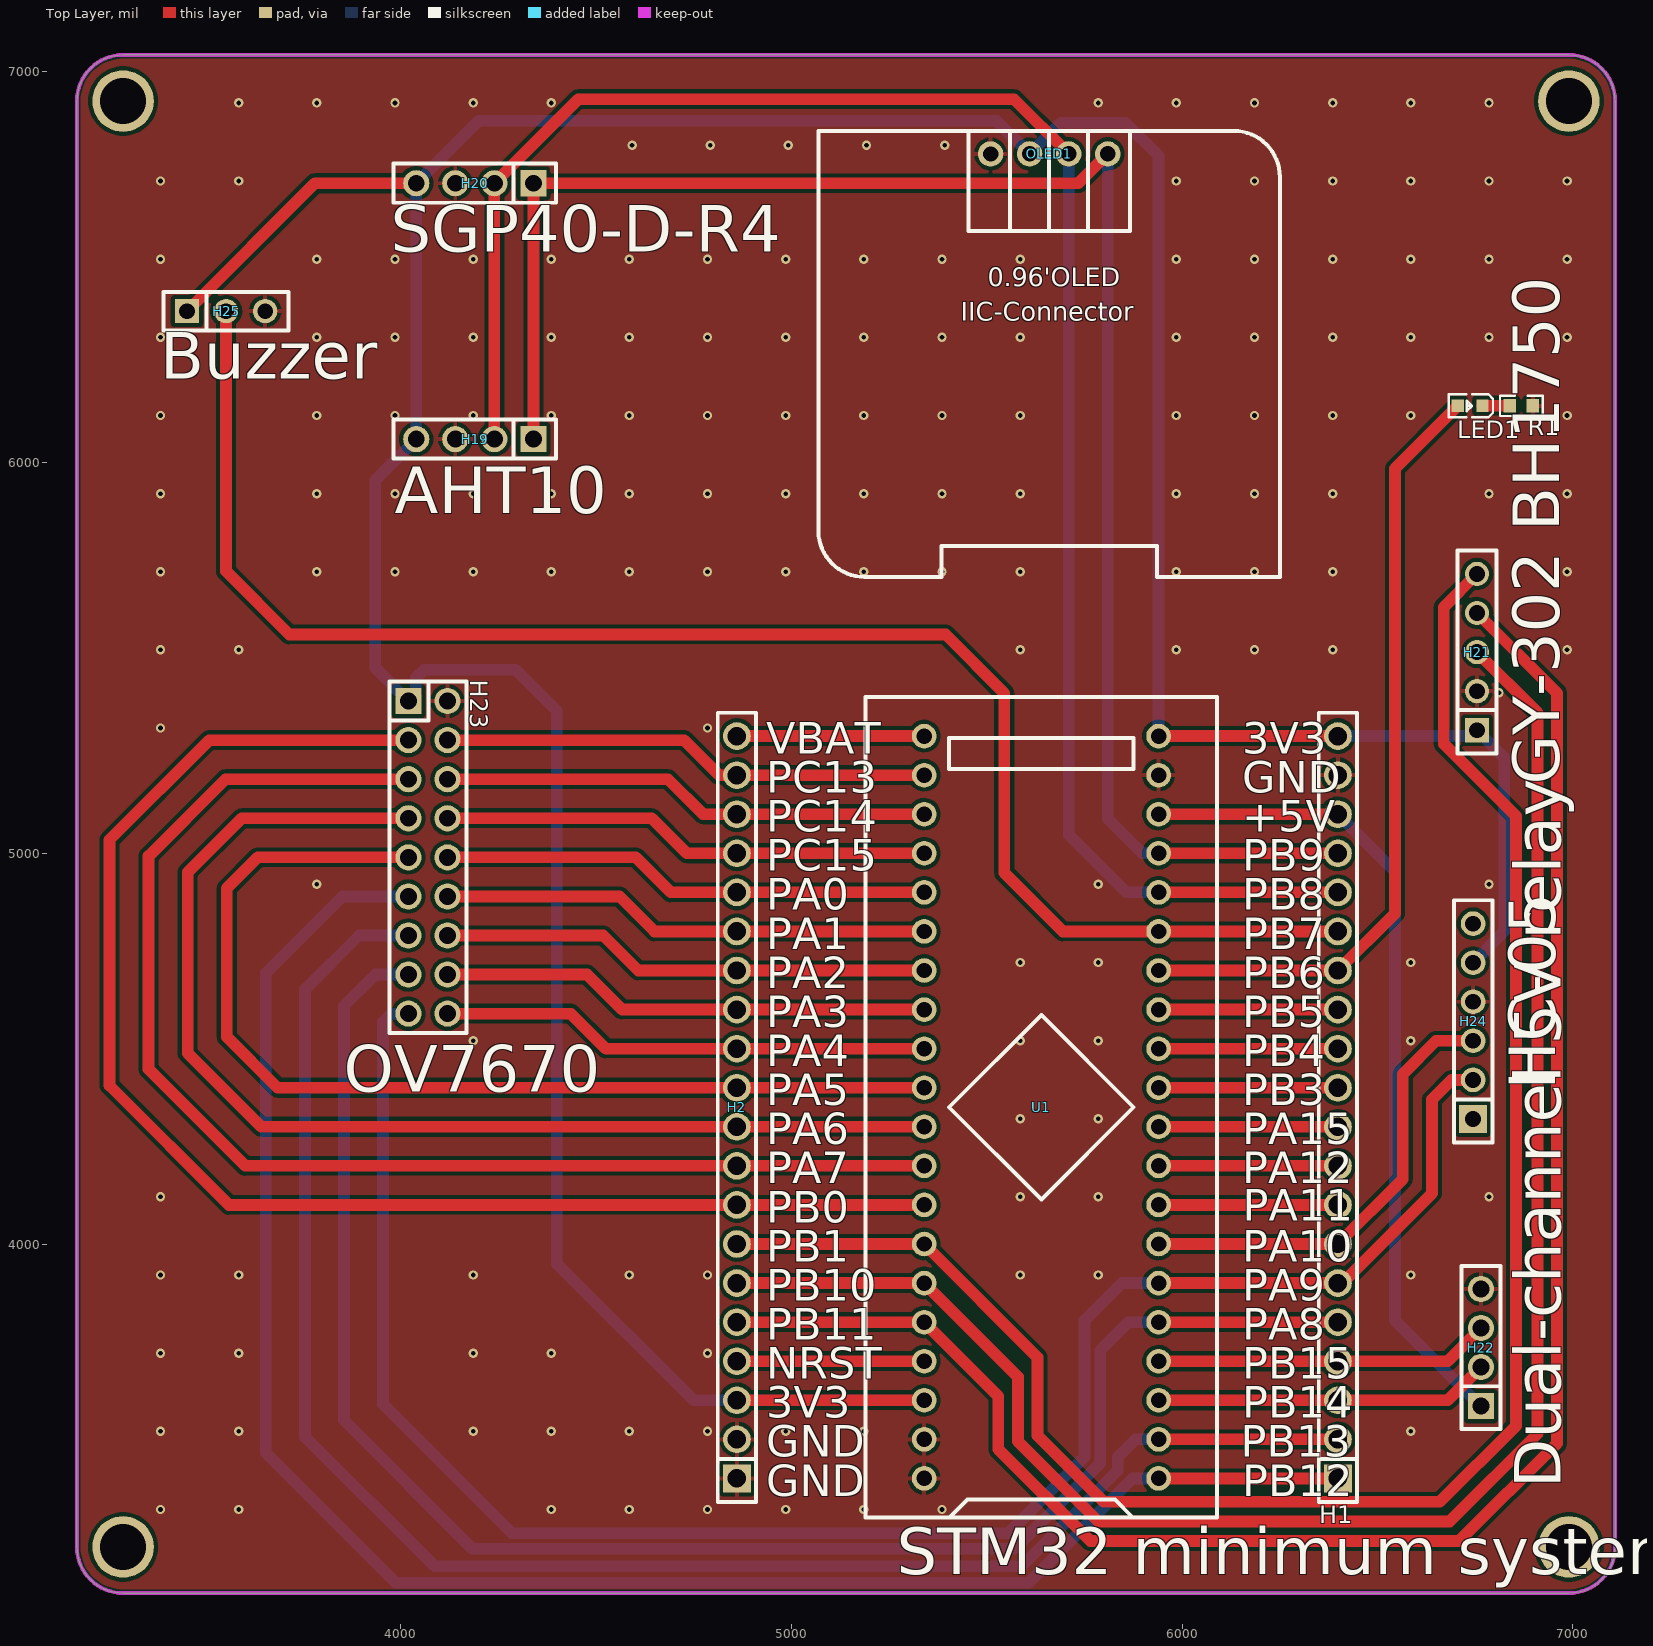
[diagram p0: Top Layer view]
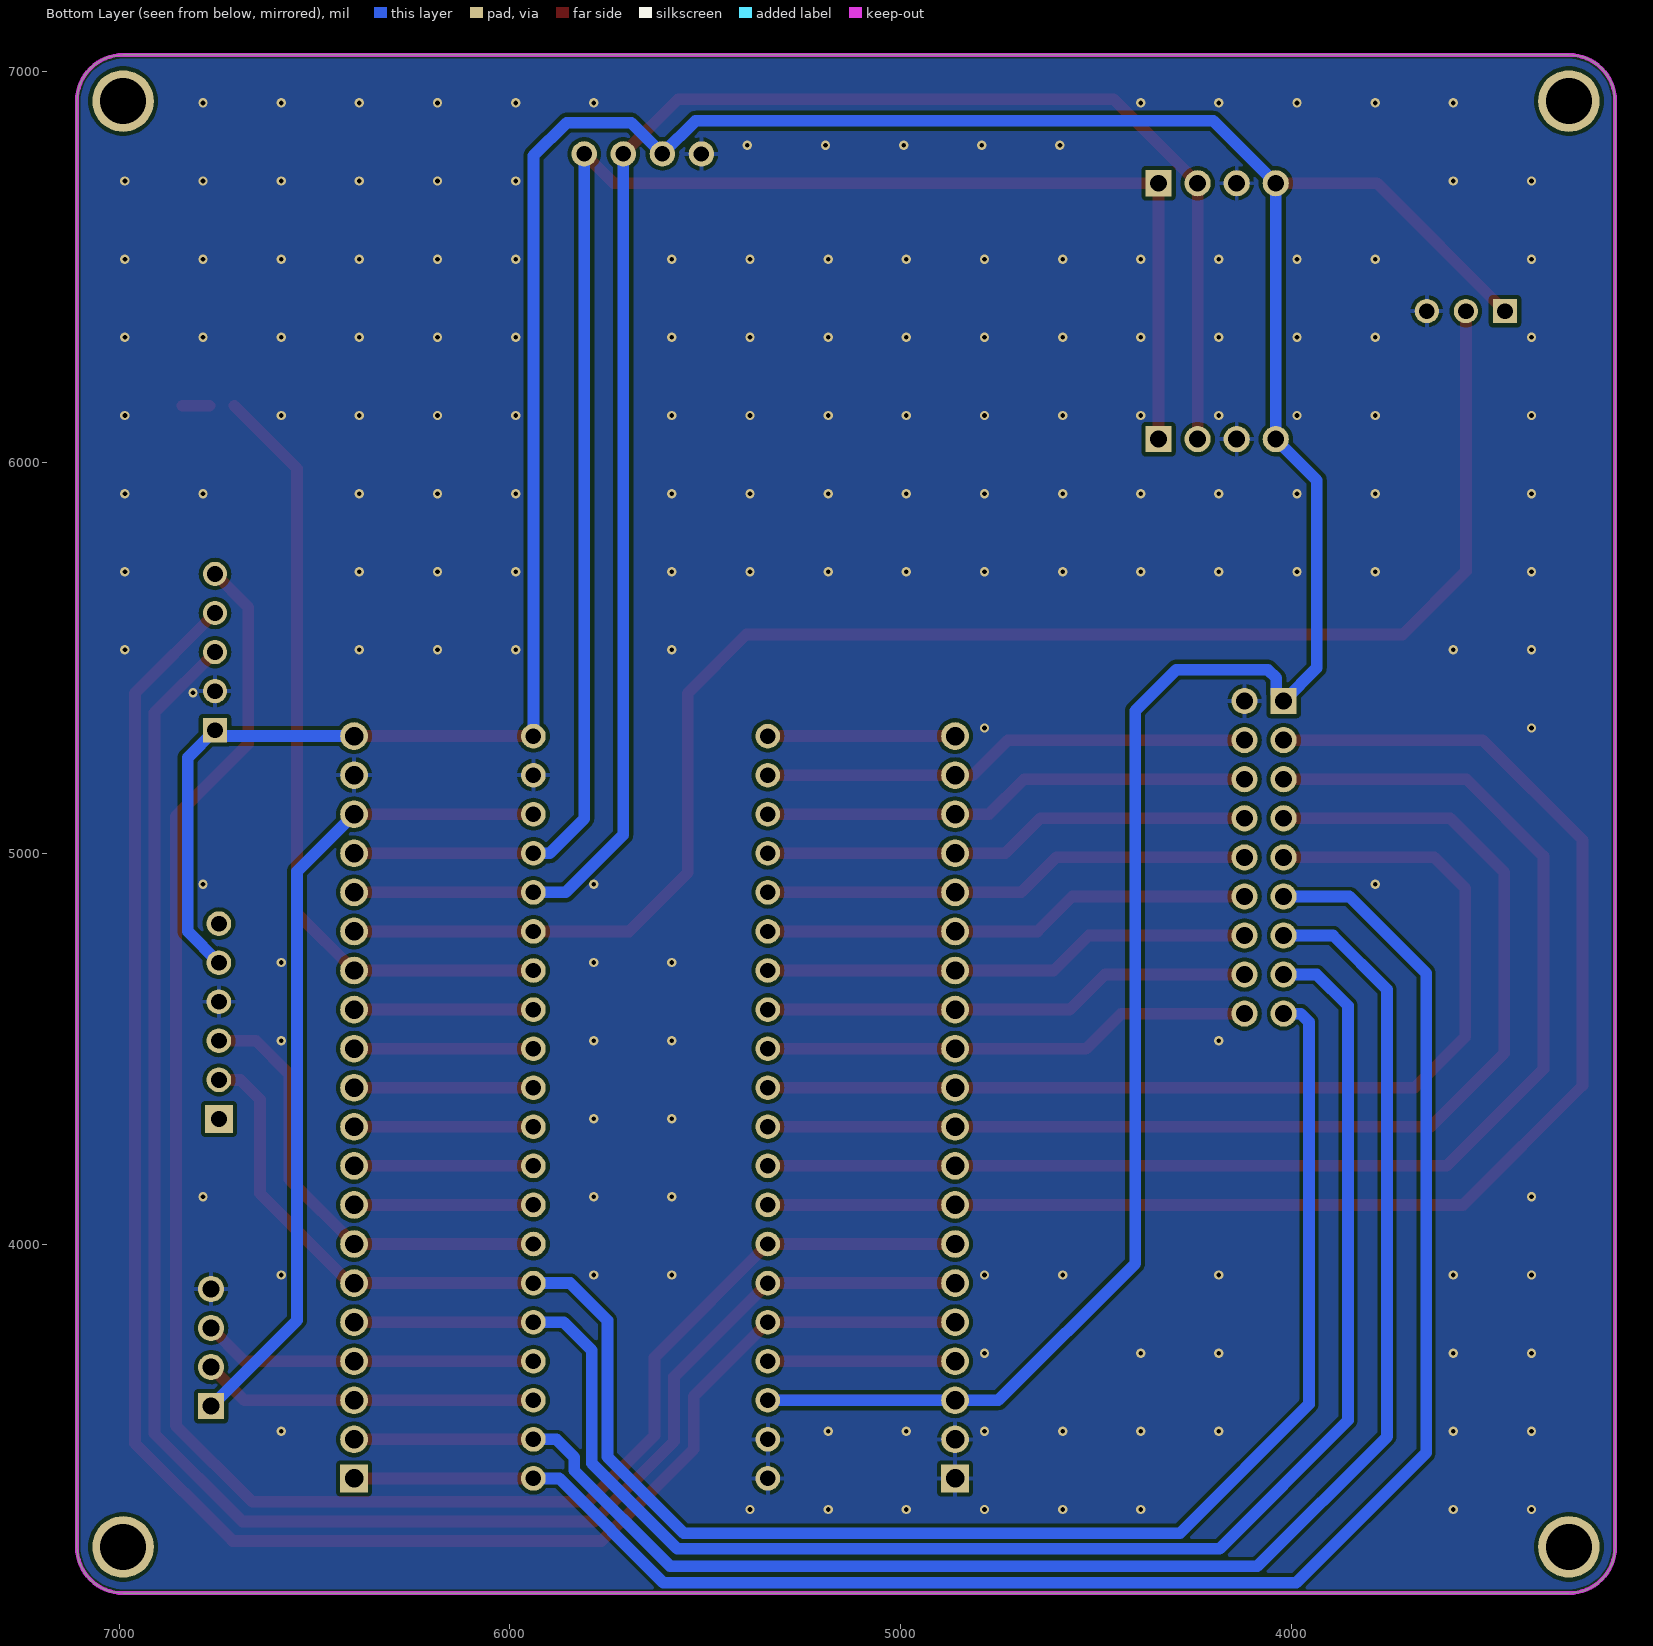
[diagram p1: Bottom Layer view, seen from below]
# Altium PCB MISC78996.pcbdoc
Units mil, origin at the board's own origin, x right, y up, seen from the top; angles counter-clockwise.
Board outline 3937.01 x 3937.01 mil, 2 copper layers (Top Layer, Bottom Layer), stack 62.206 mil thick; 13 components, 38 nets, 136 pads, 161 vias.

## Layer stack, top to bottom
Top Solder Mask Layer: solder mask 0.394, Dk 3.3
Top Layer: signal copper 1.379
Dielectric1: surface 59.449, FR4, Dk 4.5
Bottom Layer: signal copper 1.378
Bottom Solder Mask Layer: solder mask 0.394, Dk 3.3

## Board outline
3289.61,7043.5 ccw(c3289.61,6925.39) 3171.5,6925.39 3171.5,3224.61 ccw(c3289.61,3224.61) 3289.61,3106.5 6990.39,3106.5 ccw(c6990.39,3224.61) 7108.5,3224.61 7108.5,6925.39 ccw(c6990.39,6925.39) 6990.39,7043.5 3289.61,7043.5

## Design rules (kind name [scope] priority, off if disabled: settings)
BoardOutlineClearance copperThickness2oz_1 [All] p2 off: genericclearance=7.99 ignorepadtopadclearanceinfootprint=FALSE except(0: Arc-SplitContinuation Track-SplitContinuation SMDPad-SplitContinuation THPad-SplitContinuation Via-SplitContinuation Fill-SplitContinuation Region-SplitContinuation Poly-SplitContinuation Text-SplitContinuation Hole-SplitContinuation; 5.98: Arc-CutoutEdge Track-CutoutEdge SMDPad-CutoutEdge THPad-CutoutEdge Via-CutoutEdge Text-CutoutEdge; 6.9: Hole-OutlineEdge Hole-CutoutEdge; 10: Poly-OutlineEdge Poly-CutoutEdge; 11.81: Arc-OutlineEdge Track-OutlineEdge SMDPad-OutlineEdge THPad-OutlineEdge Via-OutlineEdge Fill-OutlineEdge Region-OutlineEdge Text-OutlineEdge Fill-CutoutEdge Region-CutoutEdge)
BoardOutlineClearance Plane_innerPlane_1 [All] p4 off: genericclearance=4.02 ignorepadtopadclearanceinfootprint=FALSE except(0: Arc-SplitContinuation Track-SplitContinuation SMDPad-SplitContinuation THPad-SplitContinuation Via-SplitContinuation Fill-SplitContinuation Region-SplitContinuation Poly-SplitContinuation Text-SplitContinuation Hole-SplitContinuation; 5.98: Arc-CutoutEdge Track-CutoutEdge SMDPad-CutoutEdge THPad-CutoutEdge Via-CutoutEdge Text-CutoutEdge; 6.9: Hole-OutlineEdge Hole-CutoutEdge; 10: Poly-OutlineEdge Poly-CutoutEdge; 11.81: Arc-OutlineEdge Track-OutlineEdge SMDPad-OutlineEdge THPad-OutlineEdge Via-OutlineEdge Fill-OutlineEdge Region-OutlineEdge Text-OutlineEdge Fill-CutoutEdge Region-CutoutEdge)
BoardOutlineClearance Copper_copperRegion_1 [All] p6 off: genericclearance=4.02 ignorepadtopadclearanceinfootprint=FALSE except(0: Arc-SplitContinuation Track-SplitContinuation SMDPad-SplitContinuation THPad-SplitContinuation Via-SplitContinuation Fill-SplitContinuation Region-SplitContinuation Poly-SplitContinuation Text-SplitContinuation Hole-SplitContinuation; 5.98: Arc-CutoutEdge Track-CutoutEdge SMDPad-CutoutEdge THPad-CutoutEdge Via-CutoutEdge Text-CutoutEdge; 6.9: Hole-OutlineEdge Hole-CutoutEdge; 10: Poly-OutlineEdge Poly-CutoutEdge; 11.81: Arc-OutlineEdge Track-OutlineEdge SMDPad-OutlineEdge THPad-OutlineEdge Via-OutlineEdge Fill-OutlineEdge Region-OutlineEdge Text-OutlineEdge Fill-CutoutEdge Region-CutoutEdge)
BoardOutlineClearance copperThickness1oz_1 [All] p8: genericclearance=4.02 ignorepadtopadclearanceinfootprint=FALSE except(0: Arc-SplitContinuation Track-SplitContinuation SMDPad-SplitContinuation THPad-SplitContinuation Via-SplitContinuation Fill-SplitContinuation Region-SplitContinuation Poly-SplitContinuation Text-SplitContinuation Hole-SplitContinuation; 5.98: Arc-CutoutEdge Track-CutoutEdge SMDPad-CutoutEdge THPad-CutoutEdge Via-CutoutEdge Text-CutoutEdge; 6.9: Hole-OutlineEdge Hole-CutoutEdge; 10: Poly-OutlineEdge Poly-CutoutEdge; 11.81: Arc-OutlineEdge Track-OutlineEdge SMDPad-OutlineEdge THPad-OutlineEdge Via-OutlineEdge Fill-OutlineEdge Region-OutlineEdge Text-OutlineEdge Fill-CutoutEdge Region-CutoutEdge)
Clearance copperThickness2oz [All] p1 off: gap=7.99 ignorepadtopadclearanceinfootprint=FALSE except(5.98: SMDPad-Track SMDPad-SMDPad THPad-Track SMDPad-THPad THPad-THPad Track-Via SMDPad-Via THPad-Via Via-Via Fill-SMDPad Region-SMDPad Fill-THPad Region-THPad Fill-Via Region-Via Fill-Fill Fill-Region Region-Region Arc-Track Arc-SMDPad Arc-THPad Arc-Via Fill-Arc Region-Arc Arc-Arc Text-Track SMDPad-Text Text-THPad Text-Via Fill-Text Region-Text Arc-Text Text-Text; 6.9: Hole-Track Hole-SMDPad Hole-THPad Hole-Via Fill-Hole Region-Hole Hole-Arc Hole-Text; 10: Poly-Track Poly-SMDPad Poly-THPad Poly-Via Poly-Fill Poly-Region Poly-Poly Poly-Arc Poly-Text Poly-Hole; 11.81: Fill-Track Region-Track)
Clearance Plane_innerPlane [All] p3 off: gap=4.02 ignorepadtopadclearanceinfootprint=FALSE except(5.98: SMDPad-Track SMDPad-SMDPad THPad-Track SMDPad-THPad THPad-THPad Track-Via SMDPad-Via THPad-Via Via-Via Fill-SMDPad Region-SMDPad Fill-THPad Region-THPad Fill-Via Region-Via Fill-Fill Fill-Region Region-Region Arc-Track Arc-SMDPad Arc-THPad Arc-Via Fill-Arc Region-Arc Arc-Arc Text-Track SMDPad-Text Text-THPad Text-Via Fill-Text Region-Text Arc-Text Text-Text; 6.9: Hole-Track Hole-SMDPad Hole-THPad Hole-Via Fill-Hole Region-Hole Hole-Arc Hole-Text; 10: Poly-Track Poly-SMDPad Poly-THPad Poly-Via Poly-Fill Poly-Region Poly-Poly Poly-Arc Poly-Text Poly-Hole; 11.81: Fill-Track Region-Track)
Clearance Copper_copperRegion [All] p5 off: gap=4.02 ignorepadtopadclearanceinfootprint=FALSE except(5.98: SMDPad-Track SMDPad-SMDPad THPad-Track SMDPad-THPad THPad-THPad Track-Via SMDPad-Via THPad-Via Via-Via Fill-SMDPad Region-SMDPad Fill-THPad Region-THPad Fill-Via Region-Via Fill-Fill Fill-Region Region-Region Arc-Track Arc-SMDPad Arc-THPad Arc-Via Fill-Arc Region-Arc Arc-Arc Text-Track SMDPad-Text Text-THPad Text-Via Fill-Text Region-Text Arc-Text Text-Text; 6.9: Hole-Track Hole-SMDPad Hole-THPad Hole-Via Fill-Hole Region-Hole Hole-Arc Hole-Text; 10: Poly-Track Poly-SMDPad Poly-THPad Poly-Via Poly-Fill Poly-Region Poly-Poly Poly-Arc Poly-Text Poly-Hole; 11.81: Fill-Track Region-Track)
Clearance copperThickness1oz [All] p7: gap=4.02 ignorepadtopadclearanceinfootprint=FALSE except(5.98: SMDPad-Track SMDPad-SMDPad THPad-Track SMDPad-THPad THPad-THPad Track-Via SMDPad-Via THPad-Via Via-Via Fill-SMDPad Region-SMDPad Fill-THPad Region-THPad Fill-Via Region-Via Fill-Fill Fill-Region Region-Region Arc-Track Arc-SMDPad Arc-THPad Arc-Via Fill-Arc Region-Arc Arc-Arc Text-Track SMDPad-Text Text-THPad Text-Via Fill-Text Region-Text Arc-Text Text-Text; 6.9: Hole-Track Hole-SMDPad Hole-THPad Hole-Via Fill-Hole Region-Hole Hole-Arc Hole-Text; 10: Poly-Track Poly-SMDPad Poly-THPad Poly-Via Poly-Fill Poly-Region Poly-Poly Poly-Arc Poly-Text Poly-Hole; 11.81: Fill-Track Region-Track)
DiffPairsRouting differentialPair [All] p1: maxlimit=6 minlimit=6 mostfreqgap=6 toplayer_minwidth=5 toplayer_prefwidth=10 toplayer_maxwidth=100 toplayer_mingap=6 toplayer_prefgap=6 toplayer_maxgap=6 bottomlayer_minwidth=5 bottomlayer_prefwidth=10 bottomlayer_maxwidth=100 bottomlayer_mingap=6 bottomlayer_prefgap=6 bottomlayer_maxgap=6 maxuncoupledlength=10
HoleToHoleClearance otherClearance [All] p1: gap=11.81 allowstackedmicrovias=TRUE
Length netLength [All] p1: minlimit=0 maxlimit=0
PasteMaskExpansion pasteMaskExpansion [All] p1: expansion=0
PlaneConnect innerPlane [All] p1: planeconnectstyle=Relief reliefexpansion=20 reliefentries=4 reliefconductorwidth=10 reliefairgap=10
PolygonConnect copperRegion [All] p1: connectstyle=Relief reliefconductorwidth=10 reliefentries=4 polygonreliefangle="90 Angle" airgapwidth=10 via.connectstyle=Relief via.reliefconductorwidth=10 via.reliefentries=4 via.polygonreliefangle="90 Angle" via.airgapwidth=10
RoutingVias viaSize [All] p1: holewidth=12.01 width=24.02 viastyle="Through Hole" minholewidth=11.81 minwidth=19.68 maxholewidth=248.03 maxwidth=393.7
SolderMaskExpansion solderMaskExpansion [IsVia] p1: expansion=-1000 istentingtop=TRUE
SolderMaskExpansion solderMaskExpansion [All] p2: expansion=2 istentingtop=FALSE
Width copperThickness2oz_2 [All] p1 off: maxlimit=100 minlimit=8 preferedwidth=10
Width copperThickness1oz_2 [All] p2: maxlimit=100 minlimit=5 preferedwidth=10

## Components (designator, comment, footprint, x,y, rotation, side; value= is the part's Value field where it differs from the comment)
H1 "" HDR-TH_20P-P2.54-V-F 6399.16,4350 r90 top
H2 "" HDR-TH_20P-P2.54-V-F 4860.95,4350 r90 top
H19 "" HDR-TH_4P-P2.54-V-F 4190,6060 r180 top
H20 "" HDR-TH_4P-P2.54-V-F 4190,6715 r180 top
H21 "" HDR-TH_5P-P2.54-V-F 6755,5515 r90 top
H22 "" HDR-TH_4P-P2.54-V-F 6765,3735 r90 top
H23 "" HDR-TH_18P-P2.54-V-M-R2-C9-S2.54 4069.9,4989.62 r270 top
H24 "" HDR-TH_6P-P2.54-V-F 6745,4570 r90 top
H25 "" HDR-TH_3P-P2.54-V-F 3553.37,6387.69 r0 top
LED1 "" LED_0603 6735.55,6145.2 r180 top
OLED1 "" 0.96OLED_4P 5660,6790 r0 top
R1 "510" R0603 6868.42,6145.2 r0 top
U1 "STM32F103C8T6-Card" CONN-TH_L53.3-W22.9_STM32F103C8T6-CARD 5640,4350 r90 top

## Footprints (in the part's own frame and the unit in brackets; to place one, negate y for a bottom-side part, rotate by r counter-clockwise, add the part's x,y. Pads: shape width x height; smd on the part's side, far side on the other; paste and mask are expansions set on the pad)
0.96OLED_4P [mm]
  round 1.65 hole 1 copper offset 0,0: 1(-3.81,-0.001) 2(-1.27,0.002) 3(1.27,0.002) 4(3.81,0.002)
  silkscreen extent -15,-27.5 15,1.5
CONN-TH_L53.3-W22.9_STM32F103C8T6-CARD [mm]
  round 1.6 hole 1: 1(-24.13,-7.62) 2(-21.59,-7.62) 3(-19.05,-7.62) 4(-16.51,-7.62) 5(-13.97,-7.62) 6(-11.43,-7.62) 7(-8.89,-7.62) 8(-6.35,-7.62) 9(-3.81,-7.62) 10(-1.27,-7.62) 11(1.27,-7.62) 12(3.81,-7.62) 13(6.35,-7.62) 14(8.89,-7.62) 15(11.43,-7.62) 16(13.97,-7.62) 17(16.51,-7.62) 18(19.05,-7.62) 19(21.59,-7.62) 20(24.13,-7.62) 21(24.13,7.62) 22(21.59,7.62) 23(19.05,7.62) 24(16.51,7.62) 25(13.97,7.62) 26(11.43,7.62) 27(8.89,7.62) 28(6.35,7.62) 29(3.81,7.62) 30(1.27,7.62) 31(-1.27,7.62) 32(-3.81,7.62) 33(-6.35,7.62) 34(-8.89,7.62) 35(-11.43,7.62) 36(-13.97,7.62) 37(-16.51,7.62) 38(-19.05,7.62) 39(-21.59,7.62) 40(-24.13,7.62)
  silkscreen extent -26.67,-11.43 26.67,11.43
HDR-TH_3P-P2.54-V-F [mil]
  rect 62x62 hole 40.16: 1(-100,0)
  round 62 hole 40.16: 2(0,0) 3(100,0)
  silkscreen extent -160,-49 160,49
HDR-TH_4P-P2.54-V-F [mm]
  rect 1.7x1.7 hole 1.1: 1(-3.81,0)
  round 1.7 hole 1.1: 2(-1.27,0) 3(1.27,0) 4(3.81,0)
  silkscreen extent -5.29,-1.27 5.29,1.27
HDR-TH_5P-P2.54-V-F [mil]
  rect 62x62 hole 40.16: 1(-200,0)
  round 62 hole 40.16: 2(-100,0) 3(0,0) 4(100,0) 5(200,0)
  silkscreen extent -260,-50 260,50
HDR-TH_6P-P2.54-V-F [mm]
  rect 1.8x1.8 hole 1.02: 1(-6.35,0)
  round 1.6 hole 1.02: 2(-3.81,0) 3(-1.27,0) 4(1.27,0) 5(3.81,0) 6(6.35,0)
  silkscreen extent -7.87,-1.25 7.87,1.25
HDR-TH_18P-P2.54-V-M-R2-C9-S2.54 [mm]
  rect 1.7x1.7 hole 1.1: 1(-10.16,-1.27)
  round 1.7 hole 1.1: 2(-10.16,1.27) 3(-7.62,-1.27) 4(-7.62,1.27) 5(-5.08,-1.27) 6(-5.08,1.27) 7(-2.54,-1.27) 8(-2.54,1.27) 9(0,-1.27) 10(0,1.27) 11(2.54,-1.27) 12(2.54,1.27) 13(5.08,-1.27) 14(5.08,1.27) 15(7.62,-1.27) 16(7.62,1.27) 17(10.16,-1.27) 18(10.16,1.27)
  silkscreen extent -11.43,-2.5 11.43,2.5
HDR-TH_20P-P2.54-V-F [mm]
  rect 1.8x1.8 hole 1.2: 1(-24.13,0)
  round 1.8 hole 1.2: 2(-21.59,0) 3(-19.05,0) 4(-16.51,0) 5(-13.97,0) 6(-11.43,0) 7(-8.89,0) 8(-6.35,0) 9(-3.81,0) 10(-1.27,0) 11(1.27,0) 12(3.81,0) 13(6.35,0) 14(8.89,0) 15(11.43,0) 16(13.97,0) 17(16.51,0) 18(19.05,0) 19(21.59,0) 20(24.13,0)
  silkscreen extent -25.65,-1.25 25.65,1.25
LED_0603 [mil]
  rect 31.5x31.5 smd paste+0 mask+2: 1(-33.5,-0.4) 2(29.5,-0.2)
  silkscreen extent -61,-30 53,30
R0603 [mil]
  rect 31.75x34.02 smd paste-3937.01 mask+2: 1(-29.66,0) 2(29.66,0)
  silkscreen extent -55,-26 55,26

## Free pads (board coordinates)
  round 157.48 hole 118.11: 1(3289.61,6925.39) 1(3289.61,3224.61) 1(6990.39,6925.39) 1(6990.39,3224.61)

## Via types
v1: diameter 24.02, hole 12, Top Layer to Bottom Layer, 161 vias

## Nets (pads, with @x,y where several pads share a name; then routed paths per layer and width w, separated by ;. In a path a pad name is that pad's centre, name@x,y a point inside that pad or via, vN(x,y) a via of type N, cw(c..) or ccw(c..) an arc to the next point about the centre after c; other vN are vias at no path point)
$1N17423: LED1.1 R1.1 | length 69.9
  Top Layer w30: LED1.1 6838.36,6145.6 R1.1
+5V: H1.18 H22.1 U1.18 | length 2125.7
  Top Layer w30: U1.18 H1.18
  Bottom Layer w30: H1.18 6545,4954.16 6545,3805 H22.1
GND: H1.19 H2.1 H2.2 H19.3 H20.3 H21.2 H22.4 H23.2 H24.4 H25.3 OLED1.1 R1.2 U1.19 U1.39 U1.40
  other v1: 3385.6,3320.6 3585.6,3320.6 4385.6,3320.6 4585.6,3320.6 4785.6,3320.6 4985.6,3320.6 5185.6,3320.6 5385.6,3320.6 3385.6,3520.6 3585.6,3520.6 4185.6,3520.6 4385.6,3520.6 4585.6,3520.6 4785.6,3520.6 4985.6,3520.6 5185.6,3520.6 6585.6,3520.6 3385.6,3720.6 3585.6,3720.6 4185.6,3720.6 4385.6,3720.6 4785.6,3720.6 3385.6,3920.6 3585.6,3920.6 4185.6,3920.6 4585.6,3920.6 4785.6,3920.6 5585.6,3920.6 5785.6,3920.6 6585.6,3920.6 3385.6,4120.6 5585.6,4120.6 5785.6,4120.6 6785.6,4120.6 5585.6,4320.6 5785.6,4320.6 4185.6,4520.6 5585.6,4520.6 5785.6,4520.6 6585.6,4520.6 5585.6,4720.6 5785.6,4720.6 6585.6,4720.6 3785.6,4920.6 5785.6,4920.6 6785.6,4920.6 3385.6,5320.6 4785.6,5320.6 6811.42,5410.9 3385.6,5520.6 3585.6,5520.6 5585.6,5520.6 5985.6,5520.6 6185.6,5520.6 6385.6,5520.6 6985.6,5520.6 3385.6,5720.6 3785.6,5720.6 3985.6,5720.6 4185.6,5720.6 4385.6,5720.6 4585.6,5720.6 4785.6,5720.6 4985.6,5720.6 5185.6,5720.6 5385.6,5720.6 5585.6,5720.6 5985.6,5720.6 6185.6,5720.6 6385.6,5720.6 6985.6,5720.6 3385.6,5920.6 3785.6,5920.6 3985.6,5920.6 4185.6,5920.6 4385.6,5920.6 4585.6,5920.6 4785.6,5920.6 4985.6,5920.6 5185.6,5920.6 5385.6,5920.6 5585.6,5920.6 5985.6,5920.6 6185.6,5920.6 6385.6,5920.6 6785.6,5920.6 6985.6,5920.6 3385.6,6120.6 3785.6,6120.6 3985.6,6120.6 4185.6,6120.6 4385.6,6120.6 4585.6,6120.6 4785.6,6120.6 4985.6,6120.6 5185.6,6120.6 5385.6,6120.6 5585.6,6120.6 5985.6,6120.6 6185.6,6120.6 6385.6,6120.6 6585.6,6120.6 6985.6,6120.6 3385.6,6320.6 3785.6,6320.6 3985.6,6320.6 4185.6,6320.6 4385.6,6320.6 4585.6,6320.6 4785.6,6320.6 4985.6,6320.6 5185.6,6320.6 5385.6,6320.6 5585.6,6320.6 5985.6,6320.6 6185.6,6320.6 6385.6,6320.6 6585.6,6320.6 6785.6,6320.6 6985.6,6320.6 3385.6,6520.6 3785.6,6520.6 3985.6,6520.6 4185.6,6520.6 4385.6,6520.6 4585.6,6520.6 4785.6,6520.6 4985.6,6520.6 5185.6,6520.6 5385.6,6520.6 5585.6,6520.6 5985.6,6520.6 6185.6,6520.6 6385.6,6520.6 6585.6,6520.6 6785.6,6520.6 6985.6,6520.6 3385.6,6720.6 3585.6,6720.6 5985.6,6720.6 6185.6,6720.6 6385.6,6720.6 6585.6,6720.6 6785.6,6720.6 6985.6,6720.6 4592.44,6812.44 4792.44,6812.44 4992.44,6812.44 5192.44,6812.44 5392.44,6812.44 3585.6,6920.6 3785.6,6920.6 3985.6,6920.6 4185.6,6920.6 4385.6,6920.6 5785.6,6920.6 5985.6,6920.6 6185.6,6920.6 6385.6,6920.6 6585.6,6920.6 6785.6,6920.6
NRST: H2.4 U1.37 | length 479
  Top Layer w30: H2.4 U1.37
PA0: H2.16 H23.10 U1.25 | length 1257.2
  Top Layer w30: H23.10 4601.63,4989.62 4691.25,4900 H2.16 U1.25
PA1: H2.15 H23.12 U1.26 | length 1257.2
  Top Layer w30: H23.12 4560.21,4889.62 4649.83,4800 H2.15 U1.26
PA2: H2.14 H23.14 U1.27 | length 1257.2
  Top Layer w30: H23.14 4518.79,4789.62 4608.41,4700 H2.14 U1.27
PA3: H2.13 H23.16 U1.28 | length 1257.2
  Top Layer w30: H23.16 4477.37,4689.62 4566.99,4600 H2.13 U1.28
PA4: H2.12 H23.18 U1.29 | length 1257.2
  Top Layer w30: H23.18 4435.94,4589.62 4525.57,4500 H2.12 U1.29
PA5: H2.11 H23.9 U1.30 | length 2716.7
  Top Layer w30: H23.9 3634.62,4989.62 3555,4910 3555,4530 3685,4400 H2.11 U1.30
PA6: H2.10 H23.7 U1.31 | length 3048.1
  Top Layer w30: H23.7 3593.2,5089.62 3455,4951.42 3455,4488.58 3643.58,4300 H2.10 U1.31
PA7: H2.9 H23.5 U1.32 | length 3379.5
  Top Layer w30: H23.5 3551.78,5189.62 3355,4992.84 3355,4447.16 3602.16,4200 H2.9 U1.32
PA8: H1.5 H23.15 U1.5 | length 4348.5
  Top Layer w30: U1.5 H1.5
  Bottom Layer w30: H23.15 3935.01,4689.62 3855.22,4609.83 3855.22,3548.58 4183.8,3220 5571.57,3220 5790.6,3439.03 5790.6,3728.01 5862.59,3800 U1.5
PA9: H1.6 H23.17 H24.2 U1.6 | length 4803.8
  Top Layer w30: U1.6 H1.6 6410,3900 6640,4130 6640,4370 6690,4420 H24.2
  Bottom Layer w30: H23.17 3976.43,4589.62 3955.22,4568.41 3955.22,3590 4285.22,3260 5555,3260 5750.6,3455.6 5750.6,3804.57 5846.02,3900 U1.6
PA10: H1.7 H24.3 U1.7 | length 1178.1
  Top Layer w30: U1.7 H1.7 6565,4165.84 6565,4435 6650,4520 H24.3
PA11: H1.8 U1.8 | length 459.2
  Top Layer w30: U1.8 H1.8
PA12: H1.9 U1.9 | length 459.2
  Top Layer w30: U1.9 H1.9
PA15: H1.10 U1.10 | length 459.2
  Top Layer w30: U1.10 H1.10
PB0: H2.8 H23.3 U1.33 | length 3710.8
  Top Layer w30: H23.3 3510.36,5289.62 3255,5034.26 3255,4405.74 3560.73,4100 H2.8 U1.33
PB1: H2.7 H21.5 U1.34 | length 4757.2
  Top Layer w30: H2.7 U1.34 5630,3710 5630,3510 5800,3340 6660,3340 6855,3535 6855,5095 6670,5280 6670,5630 H21.5
PB3: H1.11 U1.11 | length 459.2
  Top Layer w30: U1.11 H1.11
PB4: H1.12 U1.12 | length 459.2
  Top Layer w30: U1.12 H1.12
PB5: H1.13 U1.13 | length 459.2
  Top Layer w30: U1.13 H1.13
PB6: H1.14 LED1.2 U1.14 | length 2031.7
  Top Layer w30: U1.14 H1.14 6545,4845.84 6545,5984.35 LED1.2
PB7: H1.15 H25.2 U1.15 | length 4163.1
  Top Layer w30: H25.2 3553.37,5721.63 3715,5560 5395,5560 5545,5410 5545,4950 5695,4800 U1.15 H1.15
PB8: H1.16 H19.2 H20.2 OLED1.3 U1.16 | length 4765.1
  Top Layer w30: H19.2 H20.2 4455,6930 5570.05,6930 OLED1.3@5710,6790.05 ; U1.16 H1.16
  Bottom Layer w30: OLED1.3@5710,6790.05 5710,5047.08 5857.08,4900 U1.16
PB9: H1.17 H19.1 H20.1 OLED1.4 U1.17 | length 4483.4
  Top Layer w30: H19.1 H20.1 5734.95,6715 OLED1.4@5810,6790.05 ; U1.17 H1.17
  Bottom Layer w30: OLED1.4@5810,6790.05 5810,5088.51 5898.5,5000 U1.17
PB10: H2.6 H21.3 U1.35 | length 4555.8
  Top Layer w30: H2.6 U1.35 5580,3660 5580,3495 5785,3290 6685,3290 6910,3515 6910,5360 H21.3
PB11: H2.5 H21.4 U1.36 | length 4723.6
  Top Layer w30: H2.5 U1.36 5530,3610 5530,3475 5765,3240 6710,3240 6960,3490 6960,5410 H21.4
PB12: H1.1 H23.11 U1.1 | length 4665.3
  Top Layer w30: U1.1 H1.1
  Bottom Layer w30: H23.11 3852.17,4889.62 3655.22,4692.68 3655.22,3465.74 3987.65,3133.31 5607.48,3133.31 5874.17,3400 U1.1
PB13: H1.2 H23.13 U1.2 | length 4402.1
  Top Layer w30: U1.2 H1.2
  Bottom Layer w30: H23.13 3893.59,4789.62 3755.22,4651.25 3755.22,3507.16 4087.38,3175 5590.21,3175 5835.6,3420.39 5835.6,3454.37 5881.23,3500 U1.2
PB14: H1.3 H22.2 U1.3 | length 860.2
  Top Layer w30: U1.3 6680,3600 H22.2
PB15: H1.4 H22.3 U1.4 | length 860.2
  Top Layer w30: U1.4 H1.4 6680,3700 H22.3
PC13: H2.19 H23.4 U1.22 | length 1257.2
  Top Layer w30: H23.4 4725.89,5289.62 4815.52,5200 H2.19 U1.22
PC14: H2.18 H23.6 U1.23 | length 1257.2
  Top Layer w30: H23.6 4684.47,5189.62 4774.1,5100 H2.18 U1.23
PC15: H2.17 H23.8 U1.24 | length 1257.2
  Top Layer w30: H23.8 4643.05,5089.62 4732.67,5000 H2.17 U1.24
VBAT: H2.20 U1.21 | length 479
  Top Layer w30: H2.20 U1.21
VCC: H1.20 H2.3 H19.4 H20.4 H21.1 H23.1 H24.5 H25.1 OLED1.2 U1.20 U1.38 | length 10618.9
  Top Layer w30: H25.1 3780.68,6715 H20.4 ; H2.3 U1.38 ; U1.20 H1.20
  Bottom Layer w30: U1.38 H2.3 4750,3600 4400,3950 4400,5365 4295,5470 4060,5470 4038.79,5448.79 4038.79,5408.51 H23.1 3935,5474.52 3935,5955 H19.4 H20.4 4200,6875 5525.05,6875 5610,6790.05 5689.95,6870 5855,6870 5940,6785 U1.20 ; H1.20 6740,5300 H21.1 6825,5245 6825,4800 H24.5
pads on no net: H24.1 H24.6

## Polygon pours and split planes (outlines as drawn)
GND on Bottom Layer (solid, remove dead copper, pour order 2): 3100,7165 3100,3000 7275,3000 7275,7165
GND on Top Layer (solid, remove dead copper, pour order 0): 3000,7145 3000,3075 7385,3075 7385,7145

## Keep-outs
Board Outline Layer:
  the board outline again, w10

## Silkscreen, mask and mechanical layers (free items; w line width, h text height)
Top Silkscreen Layer:
  text "SGP40-D-R4" at 3975,6540 h120
  text "Buzzer" at 3385,6215 h120
  text "AHT10" at 3985,5870 h120
  text "VBAT" at 4935.95,5255 h80
  text "3V3" at 6154.16,5255 h80
  text "GY-302 BH1750" at 6965,5175 h120 r90
  text "PC13" at 4935.95,5155 h80
  text "GND" at 6154.16,5155 h80
  text "PC14" at 4935.95,5055 h80
  text "+5V" at 6154.16,5055 h80
  text "PC15" at 4935.95,4955 h80
  text "PB9" at 6154.16,4955 h80
  text "PA0" at 4935.95,4855 h80
  text "PB8" at 6154.16,4855 h80
  text "PA1" at 4935.95,4755 h80
  text "PB7" at 6154.16,4755 h80
  text "PA2" at 4935.95,4655 h80
  text "PB6" at 6154.16,4655 h80
  text "PA3" at 4935.95,4555 h80
  text "PB5" at 6154.16,4555 h80
  text "PA4" at 4935.95,4455 h80
  text "PB4" at 6154.16,4455 h80
  text "HC-05" at 6955,4395 h120 r90
  text "OV7670" at 3855,4390 h120
  text "PA5" at 4935.95,4355 h80
  text "PB3" at 6154.16,4355 h80
  text "PA6" at 4935.95,4255 h80
  text "PA15" at 6154.16,4255 h80
  text "PA7" at 4935.95,4155 h80
  text "PA12" at 6154.16,4155 h80
  text "PA11" at 6155.95,4060 h80
  text "PB0" at 4935.95,4055 h80
  text "PB1" at 4935.95,3955 h80
  text "PA10" at 6154.16,3955 h80
  text "PB10" at 4935.95,3855 h80
  text "PA9" at 6154.16,3855 h80
  text "PB11" at 4935.95,3755 h80
  text "PA8" at 6154.16,3755 h80
  text "NRST" at 4935.95,3655 h80
  text "PB15" at 6154.16,3655 h80
  text "3V3" at 4935.95,3555 h80
  text "PB14" at 6154.16,3555 h80
  text "GND" at 4935.95,3455 h80
  text "PB13" at 6150.95,3455 h80
  text "Dual-channel 5V relay" at 6970,3375 h120 r90
  text "GND" at 4935.95,3355 h80
  text "PB12" at 6154.16,3355 h80
  text "STM32 minimum system" at 5270,3155 h120